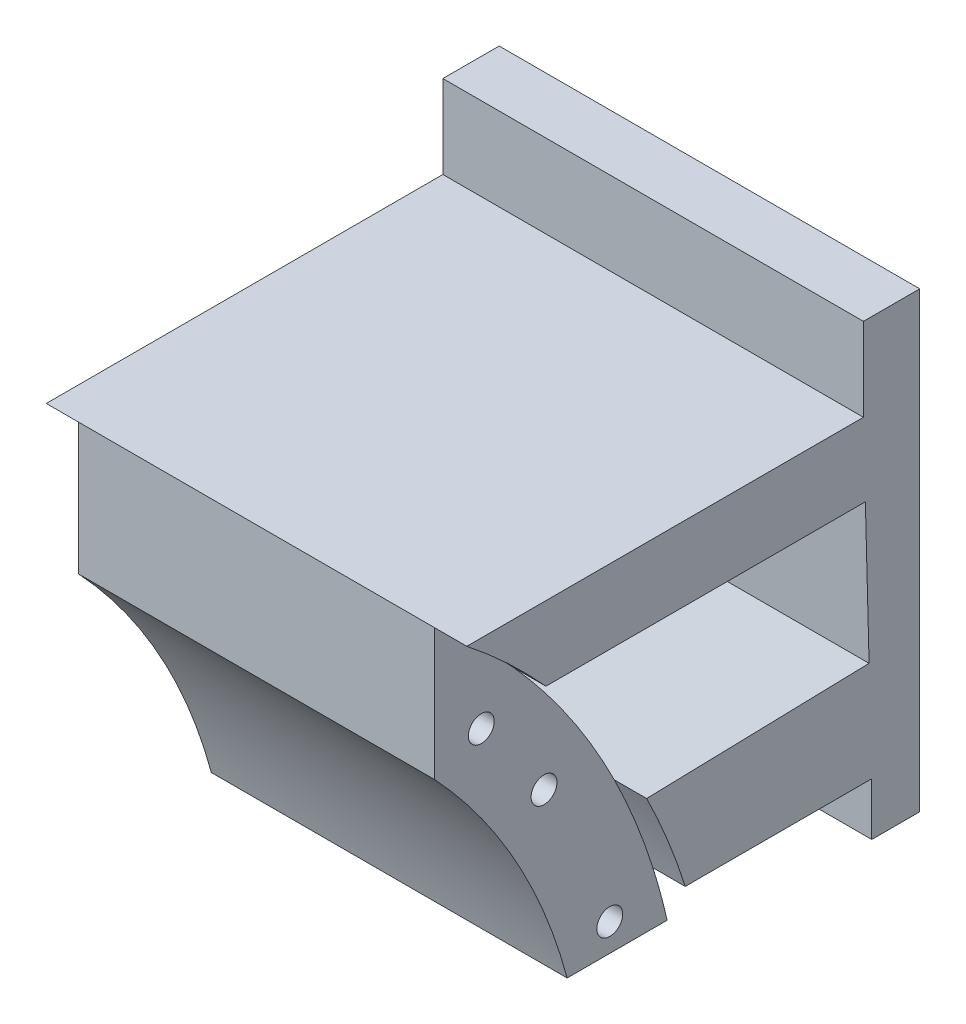
from build123d import *

# Parameters (mm, degrees)
SKETCH1_W               = 130
SKETCH1_H               = 140
BOSS_EXTRUDE1_DEPTH     = 10
SKETCH14_W              = 130
SKETCH14_H              = 140
BOSS_EXTRUDE2_DEPTH     = 130
CUT_EXTRUDE2_DEPTH      = 299.998327755
CUT_EXTRUDE2_DEPTH_BACK = 299.998327755
SKETCH15_W              = 122.59192481
SKETCH15_H              = 25.689880701
CUT_EXTRUDE4_DEPTH      = 299.998327755
CUT_EXTRUDE4_DEPTH_BACK = 10
CUT_EXTRUDE5_DEPTH      = 10
CUT_EXTRUDE6_DEPTH      = 295.78805946
CUT_EXTRUDE6_DEPTH_BACK = 295.78805946
SKETCH19_R              = 4


with BuildPart() as part:
    # Sketch1 → Boss-Extrude1 (new body)
    with BuildSketch(Plane.XY):
        with Locations((65, 160)):
            Rectangle(SKETCH1_W, SKETCH1_H)
    extrude(amount=BOSS_EXTRUDE1_DEPTH)

    # Sketch14 → Boss-Extrude2 (add)
    with BuildSketch(Plane.XY.offset(10)):
        with Locations((65, 160)):
            Rectangle(SKETCH14_W, SKETCH14_H)
    extrude(amount=BOSS_EXTRUDE2_DEPTH)

    # Sketch15 → Cut-Extrude2 (cut, two sides: drawn at the far end of the back side and taken through both)
    with BuildSketch(Plane(origin=(130, 0, 0), x_dir=(0, 0, -1), z_dir=(1, 0, 0)).offset(-CUT_EXTRUDE2_DEPTH_BACK)):
        with BuildLine():
            Line((-140, 90), (-140, 163.652960017))
            ThreePointArc((-140, 163.652960017), (-114.94393992, 129.358801446), (-98.982103949, 90))
            Line((-98.982103949, 90), (-140, 90))
        make_face()
        with BuildLine():
            Line((-68.08230106, 90), (-14.839979069, 90))
            Line((-14.839979069, 90), (-14.839979069, 106.264255909))
            Line((-14.839979069, 106.264255909), (-72.486347105, 106.264255909))
            ThreePointArc((-72.486347105, 106.264255909), (-70.115745067, 98.177775893), (-68.08230106, 90))
        make_face()
        with Locations((-78.704037595, 217.15505965)):
            Rectangle(SKETCH15_W, SKETCH15_H)
        with BuildLine():
            Line((-16.807794328, 181.392341835), (-15.660073853, 137.574182571))
            Line((-15.660073853, 137.574182571), (-84.418578186, 135.773204516))
            ThreePointArc((-84.418578186, 135.773204516), (-98.429747838, 159.645053575), (-115.553810025, 181.392341835))
            Line((-115.553810025, 181.392341835), (-16.807794328, 181.392341835))
        make_face()
    extrude(amount=CUT_EXTRUDE2_DEPTH + CUT_EXTRUDE2_DEPTH_BACK, mode=Mode.SUBTRACT)

    # Sketch17 → Cut-Extrude4 (cut, two sides: drawn at the far end of the back side and taken through both)
    with BuildSketch(Plane(origin=(130, 0, 0), x_dir=(0, 0, -1), z_dir=(1, 0, 0)).offset(-CUT_EXTRUDE4_DEPTH_BACK)):
        with BuildLine():
            Line((-140, 204.310119299), (-140, 163.652960017))
            ThreePointArc((-140, 163.652960017), (-114.94393992, 129.358801446), (-98.982103949, 90))
            Line((-98.982103949, 90), (-68.08230106, 90))
            ThreePointArc((-68.08230106, 90), (-70.115745067, 98.177775893), (-72.486347105, 106.264255909))
            ThreePointArc((-72.486347105, 106.264255909), (-98.905883629, 160.339590918), (-140, 204.310119299))
        make_face()
    extrude(amount=CUT_EXTRUDE4_DEPTH + CUT_EXTRUDE4_DEPTH_BACK, mode=Mode.SUBTRACT)

    # Sketch18 → Cut-Extrude5 (cut)
    with BuildSketch(Plane.ZY):
        with BuildLine():
            Line((98.982103949, 90), (68.08230106, 90))
            ThreePointArc((68.08230106, 90), (94.271584258, 153.301538458), (140, 204.310119299))
            Line((140, 204.310119299), (140, 163.652960017))
            ThreePointArc((140, 163.652960017), (114.94393992, 129.358801446), (98.982103949, 90))
        make_face()
    extrude(amount=-CUT_EXTRUDE5_DEPTH, mode=Mode.SUBTRACT)

    # Sketch19 → Cut-Extrude6 (cut, two sides: drawn at the far end of the back side and taken through both)
    with BuildSketch(Plane.ZY.offset(-10).offset(-CUT_EXTRUDE6_DEPTH_BACK)):
        with Locations((85.807813583, 98.537572545)):
            Circle(SKETCH19_R)
        with Locations((106.132515119, 143.973580916)):
            Circle(SKETCH19_R)
        with Locations((125.519269901, 170.036489259)):
            Circle(SKETCH19_R)
    extrude(amount=CUT_EXTRUDE6_DEPTH + CUT_EXTRUDE6_DEPTH_BACK, mode=Mode.SUBTRACT)


solid = part.part
